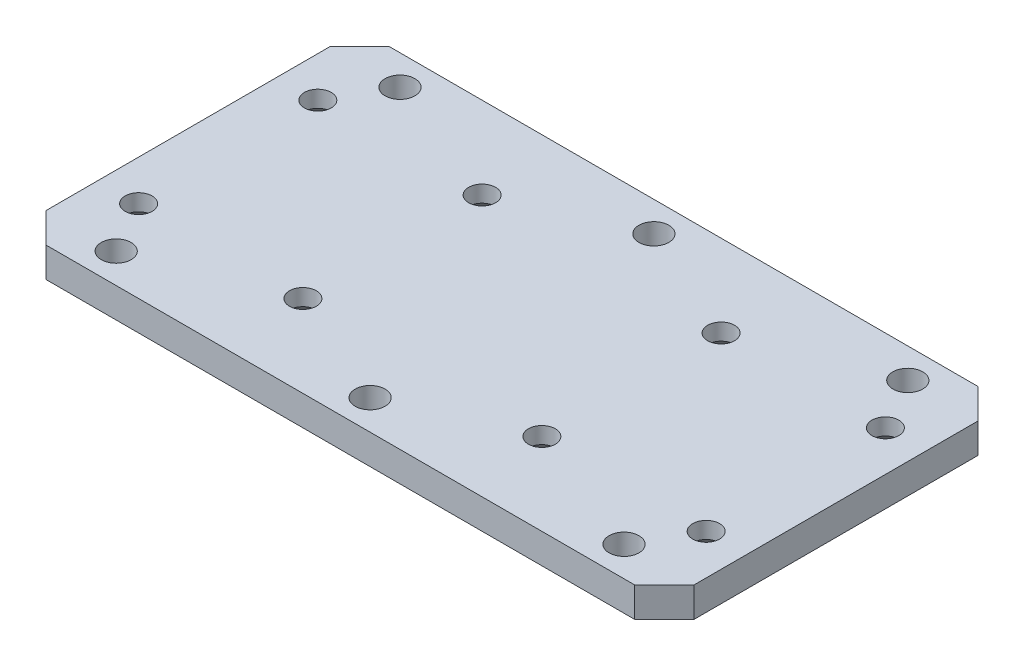
from build123d import *

# Parameters (mm, degrees)
SKETCH_1_W                   = 217
SKETCH_1_H                   = 115
EXTRUDE_1_DEPTH              = 10
HOLE_WIZARD_M8_1_D           = 9
HOLE_WIZARD_M8_1_CSINK_D     = 17.92
HOLE_WIZARD_M8_1_CSINK_ANGLE = 90
HOLE_WIZARD_M8_2_D           = 10
CHAMFER_1_SIZE               = 10


with BuildPart() as part:
    # 草图1 → 凸台-拉伸1 (new body)
    with BuildSketch(Plane(origin=(0, 0, 0), x_dir=(1, 0, 0), z_dir=(0, 1, 0))):
        Rectangle(SKETCH_1_W, SKETCH_1_H)
    extrude(amount=EXTRUDE_1_DEPTH)

    # M8 六角凹锥坑螺钉的锥形沉头孔1 (through all)
    with Locations(Plane(origin=(0, 0, 0), x_dir=(-1, 0, 0), z_dir=(0, -1, 0))):
        with Locations((-95, -30), (-40, -30), (40, -30), (95, -30), (95, 30), (40, 30), (-40, 30), (-95, 30)):
            CounterSinkHole(HOLE_WIZARD_M8_1_D / 2, HOLE_WIZARD_M8_1_CSINK_D / 2, counter_sink_angle=HOLE_WIZARD_M8_1_CSINK_ANGLE)

    # M8 间隙孔2 (through all)
    with Locations(Plane(origin=(0, 0, 0), x_dir=(-1, 0, 0), z_dir=(0, -1, 0))):
        with Locations((-85, 47.5), (0, 47.5), (85, 47.5), (85, -47.5), (0, -47.5), (-85, -47.5)):
            Hole(HOLE_WIZARD_M8_2_D / 2)

    # 倒角1
    chamfer_1_edges = [part.edges().sort_by_distance(p)[0] for p in [
        (108.5, 5, 57.5),
        (-108.5, 5, 57.5),
        (-108.5, 5, -57.5),
        (108.5, 5, -57.5),
    ]]
    chamfer(chamfer_1_edges, length=CHAMFER_1_SIZE)


solid = part.part
